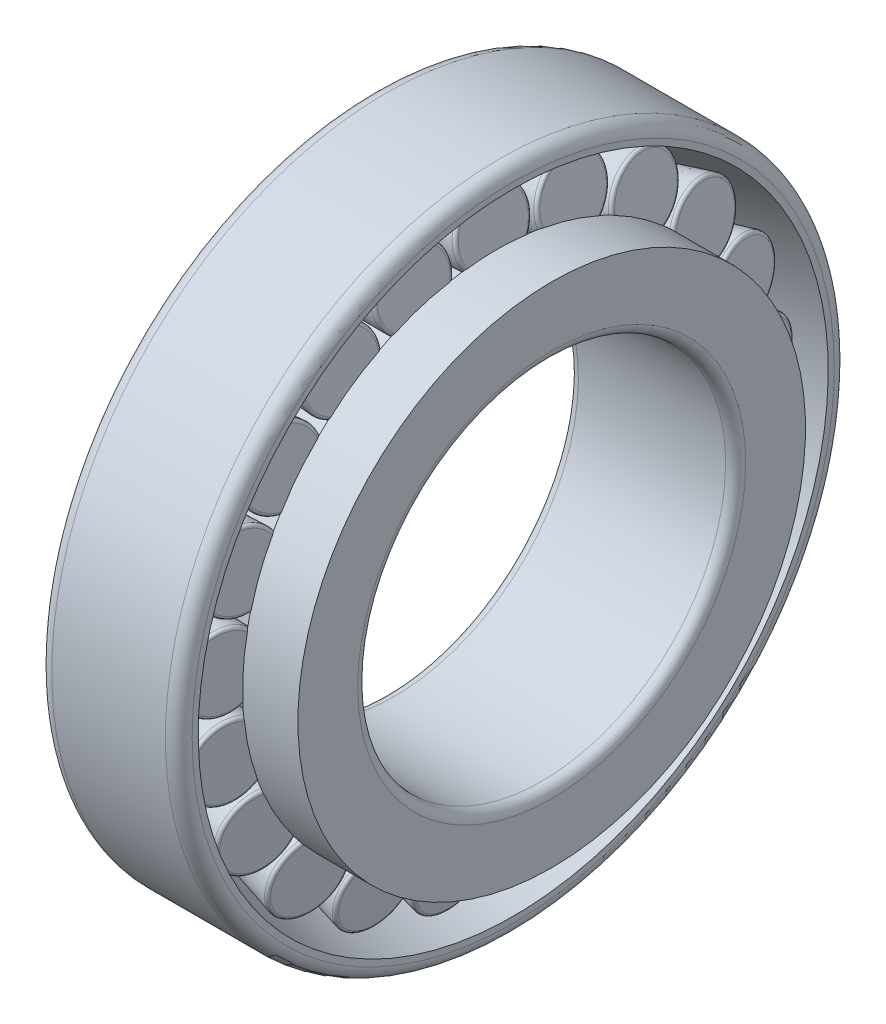
from build123d import *

# Parameters (mm, degrees)
CIRCULAR_PATTERN1_COUNT = 21


with BuildPart() as part:
    # Sketch1 → Revolve1 (revolve)
    with BuildSketch(Plane.XY):
        with BuildLine():
            Line((16.25, 37.939819746), (7.965132405, 37.939819746))
            Line((7.965132405, 37.939819746), (8.5, 34.939819746))
            Line((8.5, 34.939819746), (-5.879588575, 33.654198892))
            Line((-5.879588575, 33.654198892), (-6.147022372, 35.154198892))
            Line((-6.147022372, 35.154198892), (-8.75, 35.154198892))
            Line((-8.75, 35.154198892), (-8.75, 29))
            ThreePointArc((-8.75, 29), (-8.310660172, 27.939339828), (-7.25, 27.5))
            Line((-7.25, 27.5), (14.75, 27.5))
            ThreePointArc((14.75, 27.5), (15.810660172, 27.939339828), (16.25, 29))
            Line((16.25, 29), (16.25, 37.939819746))
        make_face()
    revolve(axis=Axis((16.25, 0, 0), (-1, 0, 0)))

    # Sketch2 → Revolve2 (revolve)
    with BuildSketch(Plane.XY):
        with BuildLine():
            Line((-6.6657338, 37.949634893), (7.53238181, 40.481005543))
            Line((7.53238181, 40.481005543), (8.437323889, 35.405307818))
            ThreePointArc((8.437323889, 35.405307818), (8.351839367, 35.053060231), (8.034382698, 34.878111011))
            Line((8.034382698, 34.878111011), (-5.485350571, 33.669366342))
            ThreePointArc((-5.485350571, 33.669366342), (-5.79868638, 33.760049025), (-5.968437439, 34.038593916))
            Line((-5.968437439, 34.038593916), (-6.6657338, 37.949634893))
        make_face()
    revolve2 = revolve(axis=Axis((-6.6657338, 37.949634893, 0), (0.9844756212878086, 0.17552136932574128, 0)))

    # Sketch3 → Revolve3 (revolve)
    with BuildSketch(Plane.XY):
        with BuildLine():
            Line((-10.5, 41.4185), (10.5, 47.08827384))
            Line((10.5, 47.08827384), (10.5, 48))
            ThreePointArc((10.5, 48), (9.914213562, 49.414213562), (8.5, 50))
            Line((8.5, 50), (-8.5, 50))
            ThreePointArc((-8.5, 50), (-9.914213562, 49.414213562), (-10.5, 48))
            Line((-10.5, 48), (-10.5, 41.4185))
        make_face()
    revolve(axis=Axis((16.25, 0, 0), (-1, 0, 0)))

    # Circular-Pattern1: Revolve2 ×21 about axis
    circular_pattern1_axis = Axis((0, 0, 0), (1, 0, 0))
    for i in range(1, CIRCULAR_PATTERN1_COUNT):
        add(revolve2.rotate(circular_pattern1_axis, i * 360 / CIRCULAR_PATTERN1_COUNT))


solid = part.part
